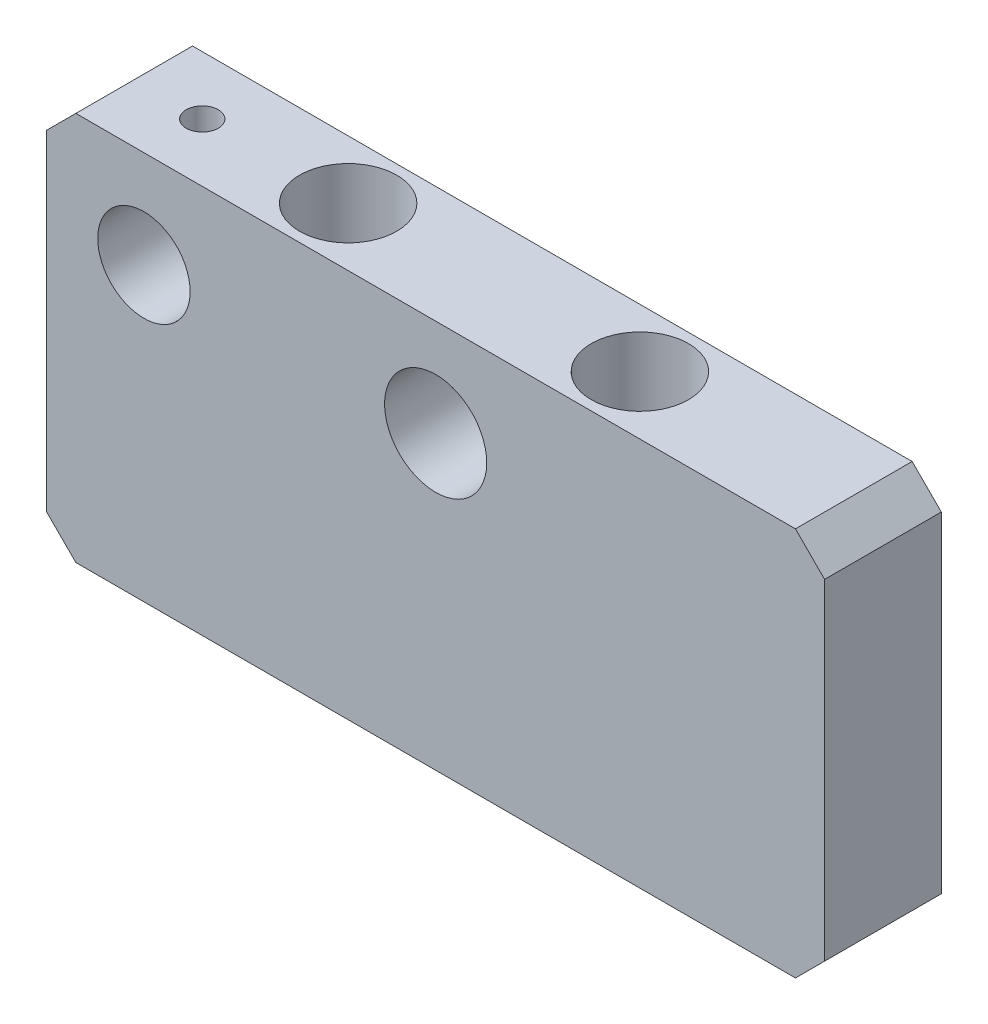
from build123d import *

# Parameters (mm, degrees)
SKETCH1_W                                           = 80
SKETCH1_H                                           = 40
BOSS_EXTRUDE1_DEPTH                                 = 12
SKETCH2_R                                           = 5.25
SKETCH2_R_2                                         = 4.75
CUT_EXTRUDE1_DEPTH                                  = 47.303347611
CBORE_FOR_M5_HEX_SOCKET_HEAD_CAP_SCREW1_D           = 5.5
CBORE_FOR_M5_HEX_SOCKET_HEAD_CAP_SCREW1_CBORE_D     = 10
CBORE_FOR_M5_HEX_SOCKET_HEAD_CAP_SCREW1_CBORE_DEPTH = 35
CHAMFER1_SIZE                                       = 3
M4_TAPPED_HOLE1_D                                   = 3.3
M4_TAPPED_HOLE1_DEPTH                               = 10.1
M4_TAPPED_HOLE1_TIP                                 = 0.991420021


with BuildPart() as part:
    # Sketch1 → Boss-Extrude1 (new body)
    with BuildSketch(Plane.XY):
        Rectangle(SKETCH1_W, SKETCH1_H)
    extrude(amount=BOSS_EXTRUDE1_DEPTH)

    # Sketch2 → Cut-Extrude1 (cut, through all)
    with BuildSketch(Plane.XY.offset(12)):
        with Locations((0, 10)):
            Circle(SKETCH2_R)
        with Locations((-30, 10)):
            Circle(SKETCH2_R_2)
    extrude(amount=-CUT_EXTRUDE1_DEPTH, mode=Mode.SUBTRACT)

    # CBORE for M5 Hex Socket Head Cap Screw1 (through all)
    with Locations(Plane(origin=(0, 20, 0), x_dir=(1, 0, 0), z_dir=(0, 1, 0))):
        with Locations((-15, -6), (15, -6)):
            CounterBoreHole(CBORE_FOR_M5_HEX_SOCKET_HEAD_CAP_SCREW1_D / 2, CBORE_FOR_M5_HEX_SOCKET_HEAD_CAP_SCREW1_CBORE_D / 2, CBORE_FOR_M5_HEX_SOCKET_HEAD_CAP_SCREW1_CBORE_DEPTH)

    # Chamfer1
    chamfer1_edges = [part.edges().sort_by_distance(p)[0] for p in [
        (40, -20, 6),
        (-40, -20, 6),
        (-40, 20, 6),
        (40, 20, 6),
    ]]
    chamfer(chamfer1_edges, length=CHAMFER1_SIZE)

    # M4 Tapped Hole1
    with Locations(Plane(origin=(0, 20, 0), x_dir=(1, 0, 0), z_dir=(0, 1, 0))):
        with Locations((-30, -6)):
            Hole(M4_TAPPED_HOLE1_D / 2, depth=M4_TAPPED_HOLE1_DEPTH)
            with Locations((0, 0, -(M4_TAPPED_HOLE1_DEPTH + M4_TAPPED_HOLE1_TIP / 2))):  # 118° drill point
                Cone(0, M4_TAPPED_HOLE1_D / 2, M4_TAPPED_HOLE1_TIP, mode=Mode.SUBTRACT)


solid = part.part
